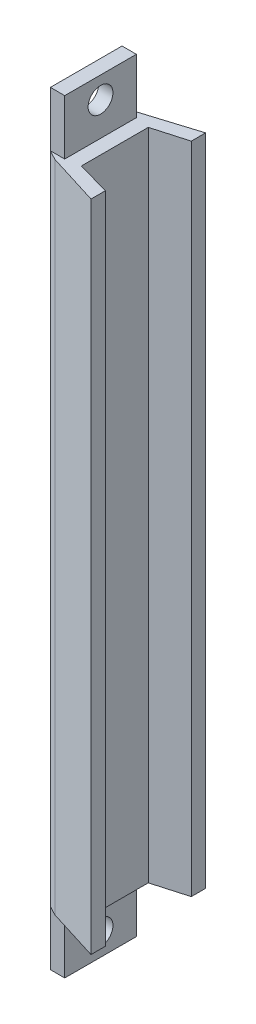
SolidWorks part; units mm, degrees
material "ZG270-500"
ref_plane "Front Plane" through (0, 0, 0) normal (0, 0, 1) x (1, 0, 0)
ref_plane "Top Plane" through (0, 0, 0) normal (0, 1, 0) x (1, 0, 0)
ref_plane "Right Plane" through (0, 0, 0) normal (1, 0, 0) x (0, 0, -1)
sketch "Sketch1" plane through (0, 0, 0) normal (0, 1, 0) x (1, 0, 0)
  line L0 (0, 0) -> (40.9343, 0) construction
  line L1 (0, -37.5) -> (0, 37.5)
  line L2 (0, 37.5) -> (10, 42.8818)
  line L3 (10, 42.8818) -> (65, 60)
  line L4 (65, 60) -> (65, 45)
  line L5 (65, 45) -> (30, 35)
  line L6 (30, 35) -> (30, -35)
  line L7 (65, -45) -> (30, -35)
  line L8 (65, -60) -> (65, -45)
  line L9 (10, -42.8818) -> (65, -60)
  line L10 (0, -37.5) -> (10, -42.8818)
  point P10 (30, 0)
  dimension "D1" = 11
  dimension "D2" = 70
  dimension "D3" = 90
  dimension "D4" = 120
  dimension "D5" = 30
  dimension "D6" = 65
  dimension "D7" = 75
  dimension "D8" = 10
extrude "Boss-Extrude1" add sketch "Sketch1" along normal mid plane 685
sketch "Sketch2" plane through (0, -342.5, 0) normal (0, -1, 0) x (1, 0, 0)
  line L8 (0, -37.5) -> (0, 37.5) construction
  line L9 (0, 37.5) -> (15, 37.5)
  line L10 (0, 37.5) -> (0, -37.5)
  line L11 (0, -37.5) -> (15, -37.5)
  line L12 (15, 37.5) -> (15, -37.5)
  line L13 (0, 0) -> (-28.0731, 0) construction
  line L14 (0, 37.5) -> (10, 42.8818) construction
  dimension "D1" = 15
extrude "Boss-Extrude2" add sketch "Sketch2" along normal blind 57.5
mirror "Mirror1" about plane through (0, 0, 0) normal (0, 1, 0) of "Boss-Extrude2"
sketch "Sketch3" plane through (0, 0, 0) normal (-1, 0, 0) x (0, 0, 1)
  line L0 (0, -377.5) -> (0, 377.5) construction
  circle A0 centre (0, 377.5) radius 13
  circle A1 centre (0, -377.5) radius 13
  point P4 (0, 0)
  dimension "D1" = 26
  dimension "D2" = 755
extrude "Cut-Extrude1" cut sketch "Sketch3" against normal blind 57.5
